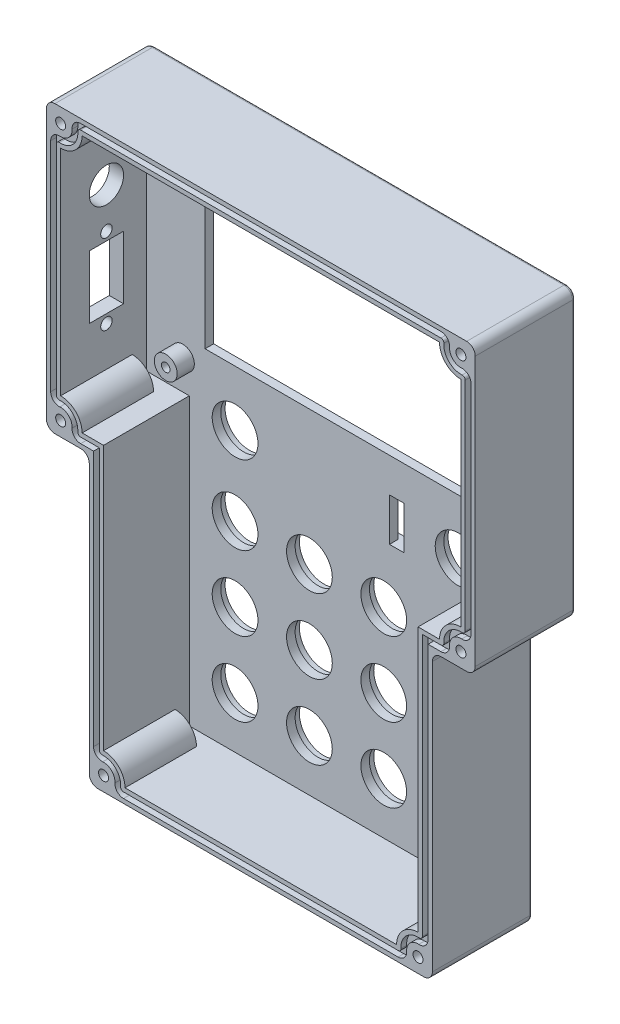
SolidWorks part; units mm, degrees
ref_plane "Front Plane" through (0, 0, 0) normal (0, 0, 1) x (1, 0, 0)
ref_plane "Top Plane" through (0, 0, 0) normal (0, 1, 0) x (1, 0, 0)
ref_plane "Right Plane" through (0, 0, 0) normal (1, 0, 0) x (0, 0, -1)
other "Configuration Table"
sketch "Sketch1" plane through (0, 0, 0) normal (0, 0, 1) x (1, 0, 0)
  line L0 (0, 0) -> (0, 200) construction
  line L1 (75, 200) -> (-75, 200)
  line L2 (-75, 200) -> (-75, 100)
  line L3 (-75, 100) -> (-60, 100)
  line L4 (-60, 100) -> (-60, 0)
  line L5 (-60, 0) -> (60, 0)
  line L6 (60, 100) -> (60, 0)
  line L7 (75, 100) -> (60, 100)
  line L8 (75, 200) -> (75, 100)
  line L10 (-49.5, 180) -> (49.5, 180)
  line L11 (-49.5, 180) -> (-49.5, 122)
  line L12 (-49.5, 122) -> (49.5, 122)
  line L13 (49.5, 180) -> (49.5, 122)
  line L14 (-49.5, 180) -> (49.5, 122) construction
  line L15 (-49.5, 122) -> (49.5, 180) construction
  circle A0 centre (-13, 23) radius 8
  circle A1 centre (-39, 23) radius 8
  circle A2 centre (-39, 49) radius 8
  circle A3 centre (-13, 49) radius 8
  circle A4 centre (-39, 75) radius 8
  circle A5 centre (-13, 75) radius 8
  circle A8 centre (-39, 102.5) radius 8
  circle A10 centre (13, 75) radius 8
  circle A11 centre (39, 75) radius 8
  circle A12 centre (13, 49) radius 8
  circle A13 centre (39, 49) radius 8
  circle A14 centre (39, 23) radius 8
  circle A15 centre (13, 23) radius 8
  circle A16 centre (39, 102.5) radius 8
  point P11 (0, 151)
  dimension "D8" = 16
  dimension "D9" = 13
  dimension "D10" = 26
  dimension "D11" = 23
  dimension "D13" = 79.5
  dimension "D1" = 150
  dimension "D2" = 200
  dimension "D3" = 100
  dimension "D4" = 120
  dimension "D5" = 99
  dimension "D6" = 58
  dimension "D7" = 49
  dimension "D12" = 3
extrude "Boss-Extrude1" add sketch "Sketch1" along normal blind 35
sketch "Sketch2" plane through (0, 0, 35) normal (0, 0, 1) x (1, 0, 0)
  line L0 (70, 105) -> (70, 195)
  line L1 (70, 195) -> (-70, 195)
  line L2 (-70, 195) -> (-70, 105)
  line L3 (-70, 105) -> (-55, 105)
  line L4 (-55, 105) -> (-55, 5)
  line L5 (-55, 5) -> (55, 5)
  line L6 (55, 5) -> (55, 105)
  line L7 (55, 105) -> (70, 105)
extrude "Cut-Extrude1" cut sketch "Sketch2" against normal blind 30
fillet "Fillet1" radius 3 8 edges at (60, 100, 17.5) (-60, 100, 17.5) (-60, 0, 17.5) (60, 0, 17.5) (75, 100, 17.5) (75, 200, 17.5) (-75, 100, 17.5) (-75, 200, 17.5)
fillet "Fillet2" radius 1 16 edges at (74.1213, 100.8787, 0) (67.5, 100, 0) (60.8787, 99.1213, 0) (60, 50, 0) (59.1213, 0.8787, 0) (0, 0, 0) (-59.1213, 0.8787, 0) (-60, 50, 0) (-60.8787, 99.1213, 0) (-67.5, 100, 0) (-74.1213, 100.8787, 0) (-75, 150, 0) (-74.1213, 199.1213, 0) (0, 200, 0) (74.1213, 199.1213, 0) (75, 150, 0)
sketch "Sketch3" plane through (0, 0, 0) normal (0, 0, -1) x (-1, 0, 0)
  line L0 (0, 122) -> (0, 58.1588) construction
  line L1 (49.5, 122) -> (-49.5, 122) construction
  circle A0 centre (-39, 23) radius 8.5
  circle A1 centre (-13, 23) radius 8.5
  circle A2 centre (-13, 49) radius 8.5
  circle A3 centre (-39, 49) radius 8.5
  circle A4 centre (-39, 75) radius 8.5
  circle A5 centre (-13, 75) radius 8.5
  circle A6 centre (-39, 102.5) radius 8.5
  circle A7 centre (39, 102.5) radius 8.5
  circle A8 centre (13, 75) radius 8.5
  circle A9 centre (39, 75) radius 8.5
  circle A10 centre (39, 49) radius 8.5
  circle A11 centre (13, 49) radius 8.5
  circle A12 centre (13, 23) radius 8.5
  circle A13 centre (39, 23) radius 8.5
  dimension "D1" = 17
extrude "Cut-Extrude2" cut sketch "Sketch3" against normal blind 2
chamfer "Chamfer1" distance 2 angle 56 4 edges at (0, 122, 0) (-49.5, 151, 0) (49.5, 151, 0) (0, 180, 0)
sketch "Sketch5" plane through (0, 0, 5) normal (0, 0, 1) x (1, 0, 0)
  line L0 (0, 180) -> (0, 98.924) construction
  line L1 (49.5, 180) -> (-49.5, 180) construction
  line L2 (72, 200) -> (-72, 200) construction
  line L3 (57.25, 115.5) -> (-57.25, 115.5) construction
  line L4 (57.25, 115.5) -> (57.25, 181.5) construction
  line L5 (57.25, 181.5) -> (-57.25, 181.5) construction
  line L6 (-57.25, 115.5) -> (-57.25, 181.5) construction
  line L7 (57.25, 115.5) -> (-57.25, 181.5) construction
  line L8 (57.25, 181.5) -> (-57.25, 115.5) construction
  circle A0 centre (-57.25, 181.5) radius 4
  circle A1 centre (-57.25, 181.5) radius 1.5
  circle A2 centre (57.25, 181.5) radius 4
  circle A3 centre (57.25, 181.5) radius 1.5
  circle A4 centre (-57.25, 115.5) radius 4
  circle A5 centre (-57.25, 115.5) radius 1.5
  circle A6 centre (57.25, 115.5) radius 4
  circle A7 centre (57.25, 115.5) radius 1.5
  point P5 (0, 148.5)
  dimension "D4" = 8
  dimension "D5" = 3
  dimension "D6" = 8
  dimension "D7" = 3
  dimension "D8" = 8
  dimension "D9" = 3
  dimension "D10" = 8
  dimension "D11" = 3
  dimension "D1" = 114.5
  dimension "D2" = 66
  dimension "D3" = 18.5
extrude "Boss-Extrude2" add sketch "Sketch5" along normal blind 6
sketch "Sketch6" plane through (0, 0, 35) normal (0, 0, 1) x (1, 0, 0)
  line L7 (-71.7471, 196.7489) -> (-62.7068, 196.7489)
  line L13 (-71.7471, 196.7489) -> (-71.7471, 187.7063)
  line L20 (71.5003, 195.7716) -> (62.5398, 195.7716)
  line L21 (71.5003, 195.7716) -> (71.5003, 187.6516)
  line L24 (71.5003, 103.14) -> (62.7343, 103.14)
  line L25 (71.5003, 103.14) -> (71.5003, 112.3484)
  line L28 (-56.4248, 4.34) -> (-47.5291, 4.34)
  line L29 (-56.4248, 4.34) -> (-56.4248, 12.3634)
  line L32 (56.3159, 4.34) -> (47.5291, 4.34)
  line L33 (56.3159, 4.34) -> (56.3159, 12.3837)
  line L36 (-71.7471, 102.6318) -> (-62.8837, 102.6318)
  line L37 (-71.7471, 102.6318) -> (-71.7471, 112.2937)
  arc A0 (62.5398, 195.7716) -> (71.5003, 187.6516) centre (70, 195) ccw
  arc A1 (71.5003, 112.3484) -> (62.7343, 103.14) centre (70, 105) ccw
  arc A2 (56.3159, 12.3837) -> (47.5291, 4.34) centre (55, 5) ccw
  arc A3 (-47.5291, 4.34) -> (-56.4248, 12.3634) centre (-55, 5) ccw
  arc A4 (-62.8837, 102.6318) -> (-71.7471, 112.2937) centre (-70, 105) ccw
  arc A5 (-71.7471, 187.7063) -> (-62.7068, 196.7489) centre (-70, 195) ccw
  dimension "D1" = 15
extrude "Boss-Extrude3" add sketch "Sketch6" against normal blind 25
sketch "Sketch7" plane through (0, 0, 35) normal (0, 0, 1) x (1, 0, 0)
  line L0 (0, 195) -> (0, 102.4209) construction
  line L1 (70, 195) -> (-70, 195) construction
  circle A0 centre (-70, 195) radius 1.75
  circle A1 centre (-70, 105) radius 1.75
  circle A2 centre (-55, 5) radius 1.75
  circle A3 centre (55, 5) radius 1.75
  circle A4 centre (70, 105) radius 1.75
  circle A5 centre (70, 195) radius 1.75
  dimension "D1" = 3.5
extrude "Cut-Extrude4" cut sketch "Sketch7" against normal blind 20
sketch "Sketch9" plane through (0, 0, 35) normal (0, 0, 1) x (1, 0, 0)
  line L0 (-70, 187.5) -> (-70, 112.5) construction
  line L1 (-62.5, 105) -> (-55, 105) construction
  line L2 (-55, 105) -> (-55, 12.5) construction
  line L3 (-47.5, 5) -> (47.5, 5) construction
  line L4 (55, 5) -> (55, 105) construction
  line L5 (55, 12.5) -> (55, 105) construction
  line L6 (55, 105) -> (62.5, 105) construction
  line L7 (55, 105) -> (70, 105) construction
  line L8 (70, 112.5) -> (70, 187.5) construction
  line L9 (70, 105) -> (70, 195) construction
  line L10 (70, 112.5) -> (70, 187.5) construction
  line L11 (62.5, 195) -> (-62.5, 195) construction
  line L12 (71.5, 111.9821) -> (71.5, 188.0179)
  line L13 (63.0179, 196.5) -> (-63.0179, 196.5)
  line L14 (-71.5, 188.0179) -> (-71.5, 111.9821)
  line L15 (-63.0179, 103.5) -> (-56.5, 103.5)
  line L16 (-56.5, 103.5) -> (-56.5, 11.9821)
  line L17 (-48.0179, 3.5) -> (48.0179, 3.5)
  line L18 (56.5, 11.9821) -> (56.5, 103.5)
  line L19 (56.5, 103.5) -> (63.0179, 103.5)
  line L20 (-71.5, 189.1905) -> (-71.5, 110.8095) construction
  line L21 (-64.1905, 103.5) -> (-56.5, 103.5) construction
  line L22 (-56.5, 103.5) -> (-56.5, 10.8095) construction
  line L23 (-49.1905, 3.5) -> (49.1905, 3.5) construction
  line L24 (56.5, 10.8095) -> (56.5, 103.5) construction
  line L25 (71.5, 110.8095) -> (71.5, 189.1905) construction
  line L26 (56.5, 103.5) -> (64.1905, 103.5) construction
  line L27 (64.1905, 196.5) -> (-64.1905, 196.5) construction
  line L28 (63.0179, 198.5) -> (-63.0179, 198.5)
  line L29 (-73.5, 188.0179) -> (-73.5, 111.9821)
  line L30 (-63.0179, 101.5) -> (-58.5, 101.5)
  line L31 (-58.5, 101.5) -> (-58.5, 11.9821)
  line L32 (-48.0179, 1.5) -> (48.0179, 1.5)
  line L33 (58.5, 11.9821) -> (58.5, 101.5)
  line L34 (58.5, 101.5) -> (63.0179, 101.5)
  line L35 (73.5, 111.9821) -> (73.5, 188.0179)
  arc A0 (-70, 112.5) -> (-62.5, 105) centre (-70, 105) cw construction
  arc A1 (-55, 12.5) -> (-47.5, 5) centre (-55, 5) cw construction
  arc A2 (47.5, 5) -> (55, 12.5) centre (55, 5) cw construction
  arc A3 (55, 12.5) -> (47.5, 5) centre (55, 5) ccw construction
  arc A4 (62.5, 195) -> (70, 187.5) centre (70, 195) ccw construction
  arc A5 (70, 112.5) -> (62.5, 105) centre (70, 105) ccw construction
  arc A6 (62.5, 195) -> (70, 187.5) centre (70, 195) ccw construction
  arc A7 (-62.5, 195) -> (-70, 187.5) centre (-70, 195) cw construction
  arc A8 (64.0153, 195.4286) -> (70.4286, 189.0153) centre (70, 195) ccw
  arc A9 (-64.0153, 195.4286) -> (-70.4286, 189.0153) centre (-70, 195) cw
  arc A10 (-70.4286, 110.9847) -> (-64.0153, 104.5714) centre (-70, 105) cw
  arc A11 (-55.4286, 10.9847) -> (-49.0153, 4.5714) centre (-55, 5) cw
  arc A12 (49.0153, 4.5714) -> (55.4286, 10.9847) centre (55, 5) cw
  arc A13 (70.4286, 110.9847) -> (64.0153, 104.5714) centre (70, 105) ccw
  arc A14 (-71.5, 110.8095) -> (-64.1905, 103.5) centre (-70, 105) cw construction
  arc A15 (-71.5, 111.9821) -> (-70.4286, 110.9847) centre (-70.5, 111.9821) ccw
  arc A16 (-64.0153, 104.5714) -> (-63.0179, 103.5) centre (-63.0179, 104.5) ccw
  arc A17 (-56.5, 10.8095) -> (-49.1905, 3.5) centre (-55, 5) cw construction
  arc A18 (-56.5, 11.9821) -> (-55.4286, 10.9847) centre (-55.5, 11.9821) ccw
  arc A19 (-49.0153, 4.5714) -> (-48.0179, 3.5) centre (-48.0179, 4.5) ccw
  arc A20 (49.1905, 3.5) -> (56.5, 10.8095) centre (55, 5) cw construction
  arc A21 (48.0179, 3.5) -> (49.0153, 4.5714) centre (48.0179, 4.5) ccw
  arc A22 (55.4286, 10.9847) -> (56.5, 11.9821) centre (55.5, 11.9821) ccw
  arc A23 (71.5, 110.8095) -> (64.1905, 103.5) centre (70, 105) ccw construction
  arc A24 (71.5, 111.9821) -> (70.4286, 110.9847) centre (70.5, 111.9821) cw
  arc A25 (63.0179, 103.5) -> (64.0153, 104.5714) centre (63.0179, 104.5) ccw
  arc A26 (64.1905, 196.5) -> (71.5, 189.1905) centre (70, 195) ccw construction
  arc A27 (71.5, 188.0179) -> (70.4286, 189.0153) centre (70.5, 188.0179) ccw
  arc A28 (64.0153, 195.4286) -> (63.0179, 196.5) centre (63.0179, 195.5) ccw
  arc A29 (-64.1905, 196.5) -> (-71.5, 189.1905) centre (-70, 195) cw construction
  arc A30 (-63.0179, 196.5) -> (-64.0153, 195.4286) centre (-63.0179, 195.5) ccw
  arc A31 (-70.4286, 189.0153) -> (-71.5, 188.0179) centre (-70.5, 188.0179) ccw
  arc A32 (-63.0179, 198.5) -> (-66.0102, 195.2857) centre (-63.0179, 195.5) ccw
  arc A33 (-66.0102, 195.2857) -> (-70.2857, 191.0102) centre (-70, 195) cw
  arc A34 (-70.2857, 191.0102) -> (-73.5, 188.0179) centre (-70.5, 188.0179) ccw
  arc A35 (-73.5, 111.9821) -> (-70.2857, 108.9898) centre (-70.5, 111.9821) ccw
  arc A36 (-70.2857, 108.9898) -> (-66.0102, 104.7143) centre (-70, 105) cw
  arc A37 (-66.0102, 104.7143) -> (-63.0179, 101.5) centre (-63.0179, 104.5) ccw
  arc A38 (-58.5, 11.9821) -> (-55.2857, 8.9898) centre (-55.5, 11.9821) ccw
  arc A39 (-55.2857, 8.9898) -> (-51.0102, 4.7143) centre (-55, 5) cw
  arc A40 (-51.0102, 4.7143) -> (-48.0179, 1.5) centre (-48.0179, 4.5) ccw
  arc A41 (48.0179, 1.5) -> (51.0102, 4.7143) centre (48.0179, 4.5) ccw
  arc A42 (51.0102, 4.7143) -> (55.2857, 8.9898) centre (55, 5) cw
  arc A43 (55.2857, 8.9898) -> (58.5, 11.9821) centre (55.5, 11.9821) ccw
  arc A44 (63.0179, 101.5) -> (66.0102, 104.7143) centre (63.0179, 104.5) ccw
  arc A45 (70.2857, 108.9898) -> (66.0102, 104.7143) centre (70, 105) ccw
  arc A46 (73.5, 111.9821) -> (70.2857, 108.9898) centre (70.5, 111.9821) cw
  arc A47 (73.5, 188.0179) -> (70.2857, 191.0102) centre (70.5, 188.0179) ccw
  arc A48 (66.0102, 195.2857) -> (70.2857, 191.0102) centre (70, 195) ccw
  arc A49 (66.0102, 195.2857) -> (63.0179, 198.5) centre (63.0179, 195.5) ccw
  dimension "D2" = 1
  dimension "D1" = 1.5
  dimension "D3" = 2
extrude "Cut-Extrude5" cut sketch "Sketch9" against normal blind 2
sketch "Sketch10" plane through (0, 0, 0) normal (0, 0, -1) x (-1, 0, 0)
  line L0 (0, 0) -> (0, 148.6871) construction
  line L1 (57, 0) -> (-57, 0) construction
  line L2 (-20, 110) -> (20, 110)
  line L3 (-20, 110) -> (-20, 95)
  line L4 (-20, 95) -> (20, 95)
  line L5 (20, 110) -> (20, 95)
  line L6 (-20, 110) -> (20, 95) construction
  line L7 (-20, 95) -> (20, 110) construction
  point P3 (0, 102.5)
  dimension "D1" = 40
  dimension "D2" = 15
  dimension "D3" = 95
extrude "Cut-Extrude6" cut sketch "Sketch10" against normal blind 2
sketch "Sketch11" plane through (0, 0, 2) normal (0, 0, -1) x (-1, 0, 0)
  line L0 (-20, 95) -> (20, 95) construction
  line L1 (-20, 110) -> (-15, 110)
  line L2 (-20, 110) -> (-20, 95)
  line L3 (-20, 95) -> (-15, 95)
  line L4 (-15, 110) -> (-15, 95)
  dimension "D1" = 5
extrude "Cut-Extrude7" cut sketch "Sketch11" against normal up to next
sketch "Sketch12" plane through (-75, 0, 0) normal (-1, 0, 0) x (0, 0, 1)
  line L0 (0, 103) -> (0, 197) construction
  line L1 (1, 200) -> (35, 200) construction
  line L2 (19, 154.38) -> (19, 126.38) construction
  line L3 (13, 151.38) -> (25, 151.38)
  line L4 (13, 151.38) -> (13, 129.38)
  line L5 (13, 129.38) -> (25, 129.38)
  line L6 (25, 151.38) -> (25, 129.38)
  circle A0 centre (19, 168.38) radius 6
  circle A1 centre (19, 154.38) radius 2
  circle A2 centre (19, 126.38) radius 2
  dimension "D1" = 19
  dimension "D2" = 31.62
  dimension "D3" = 12
  dimension "D8" = 4
  dimension "D9" = 3
  dimension "D10" = 3
  dimension "D4" = 12
  dimension "D5" = 22
  dimension "D6" = 48.62
  dimension "D7" = 13
extrude "Cut-Extrude8" cut sketch "Sketch12" against normal up to next
